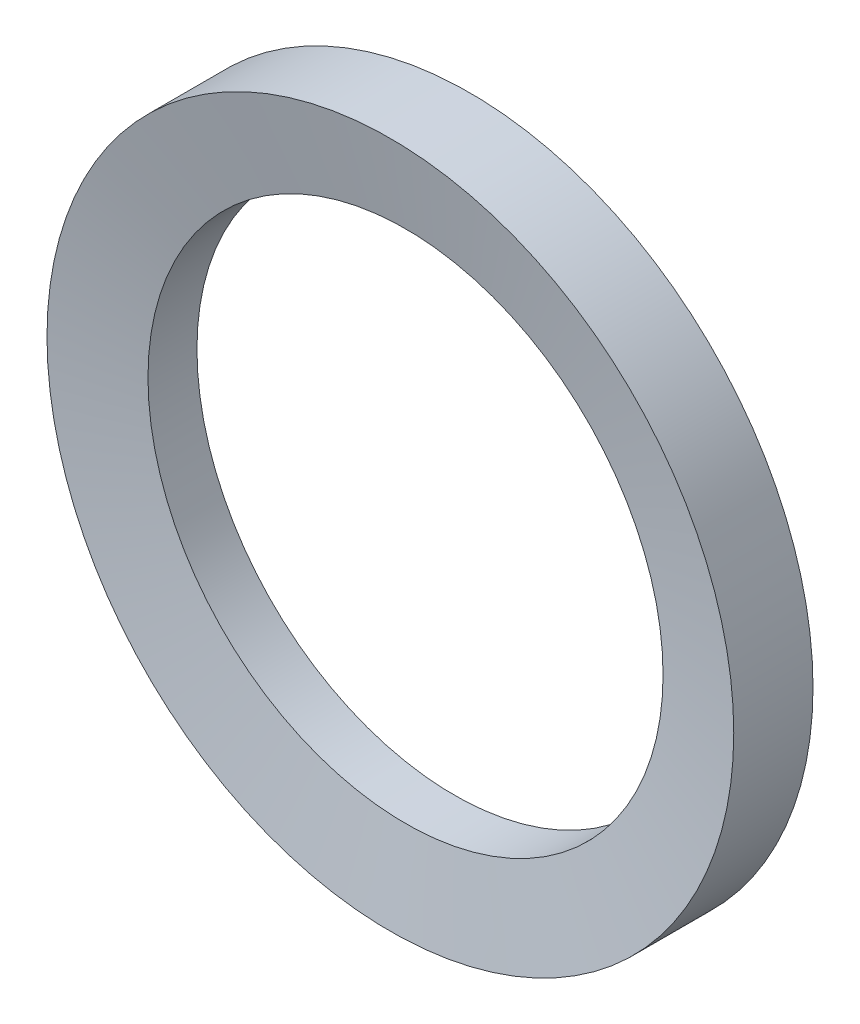
SolidWorks part; units mm, degrees
ref_plane "Front Plane" through (0, 0, 0) normal (0, 0, 1) x (1, 0, 0)
ref_plane "Top Plane" through (0, 0, 0) normal (0, 1, 0) x (1, 0, 0)
ref_plane "Right Plane" through (0, 0, 0) normal (1, 0, 0) x (0, 0, -1)
other "Configuration Table"
sketch "Sketch1" plane through (0, 0, 0) normal (0, 0, 1) x (1, 0, 0)
  circle A0 centre (0, 0) radius 19.5
  circle A1 centre (0, 0) radius 26
  dimension "D1" = 52
  dimension "D2" = 39
extrude "Boss-Extrude1" add sketch "Sketch1" along normal mid plane 6
sketch "Sketch2" plane through (0, 0, 3) normal (0, 0, 1) x (1, 0, 0)
  circle A1 centre (0, 0) radius 26 construction
  circle A2 centre (0, 0) radius 26
extrude "Cut-Extrude1" cut sketch "Sketch2" against normal blind 6 draft 80
mirror "Mirror1" about plane through (0, 0, 0) normal (0, 0, 1) of "Cut-Extrude1"
